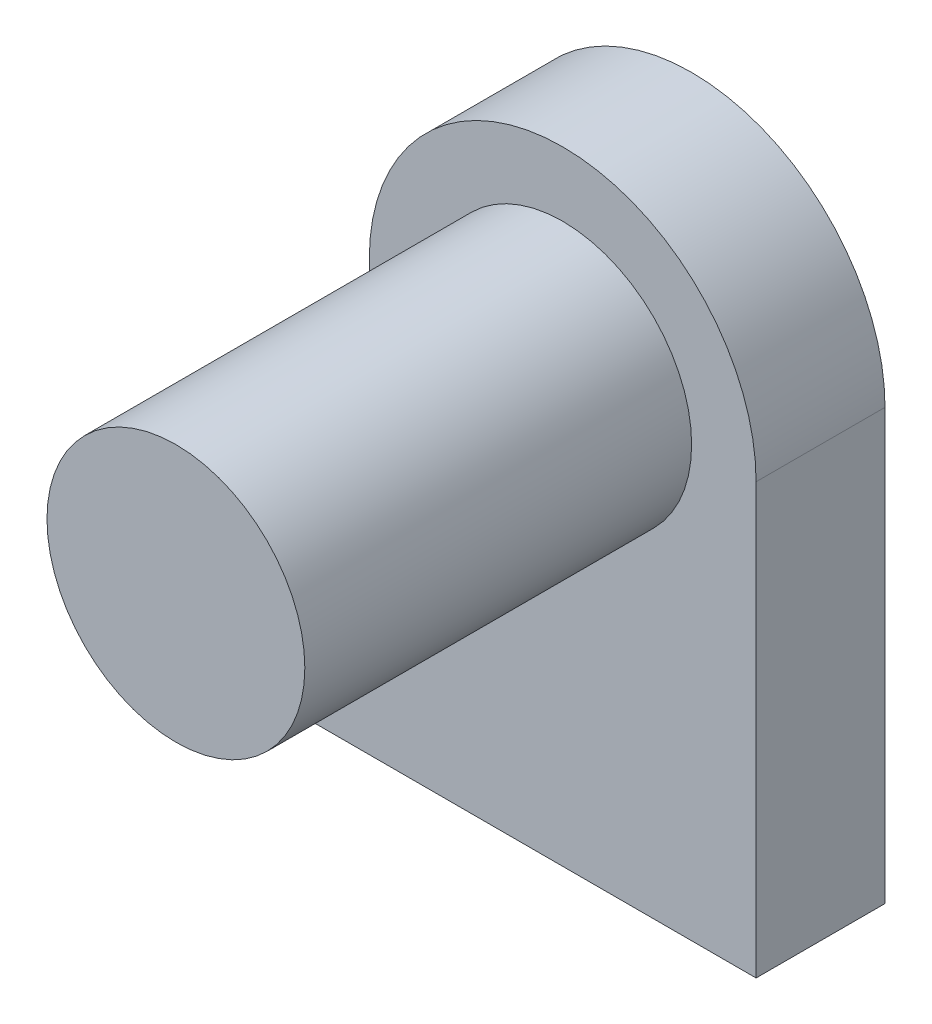
SolidWorks part; units mm, degrees
ref_plane "Front Plane" through (0, 0, 0) normal (0, 0, 1) x (1, 0, 0)
ref_plane "Top Plane" through (0, 0, 0) normal (0, 1, 0) x (1, 0, 0)
ref_plane "Right Plane" through (0, 0, 0) normal (1, 0, 0) x (0, 0, -1)
sketch "Sketch2" plane through (0, 0, 0) normal (0, 0, 1) x (1, 0, 0)
  line L1 (-75, 12.5) -> (75, 12.5)
  line L2 (-75, 12.5) -> (-75, -12.5)
  line L3 (-75, -12.5) -> (75, -12.5)
  line L4 (75, 12.5) -> (75, -12.5)
  line L5 (-75, 12.5) -> (75, -12.5) construction
  line L6 (-75, -12.5) -> (75, 12.5) construction
  point P0 (0, 0)
  dimension "D1" = 150
  dimension "D2" = 25
extrude "Boss-Extrude1" add sketch "Sketch2" along normal mid plane 30
sketch "Sketch3" plane through (0, 0, 15) normal (0, 0, 1) x (1, 0, 0)
  line L0 (75, -12.5) -> (75, 12.5) construction
  line L1 (-75, -12.5) -> (75, -12.5) construction
  line L2 (-15, 87.5) -> (-15, 0)
  line L3 (-15, 0) -> (75, 0)
  line L4 (75, 0) -> (75, 87.5)
  circle A0 centre (30, 87.5) radius 30
  arc A1 (75, 87.5) -> (-15, 87.5) centre (30, 87.5) ccw
  dimension "D1" = 60
  dimension "D2" = 90
  dimension "D3" = 100
extrude "Boss-Extrude2" add sketch "Sketch3" against normal up to surface (30 mm away) up to face at (0, 0, -15)
sketch "Sketch4" plane through (0, 12.5, 0) normal (0, 1, 0) x (1, 0, 0)
  line L0 (-75, -15) -> (-75, 15) construction
  circle A0 centre (-60, 0) radius 5.5
  circle A1 centre (-40, 0) radius 5.5
  dimension "D3" = 11
  dimension "D1" = 20
  dimension "D2" = 15
extrude "Cut-Extrude1" cut sketch "Sketch4" against normal blind 30
sketch "Sketch5" plane through (0, 0, -15) normal (0, 0, -1) x (-1, 0, 0)
  circle A0 centre (-30, 87.5) radius 30 construction
  circle A1 centre (-30, 87.5) radius 30
extrude "Boss-Extrude3" add sketch "Sketch5" against normal blind 120
